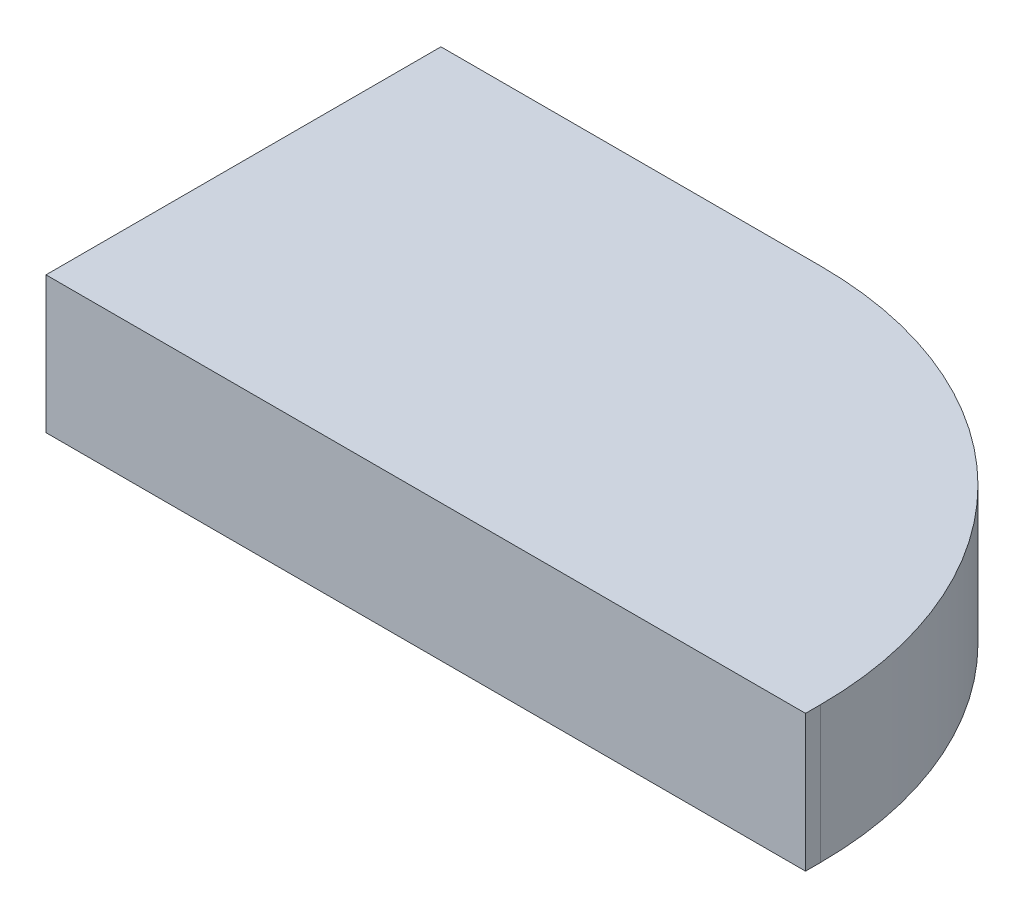
from build123d import *

# Parameters (mm, degrees)
BOSS_EXTRUDE1_DEPTH = 2.25


with BuildPart() as part:
    # Sketch1 → Boss-Extrude1 (new, symmetric)
    with BuildSketch(Plane(origin=(0, 0, 0), x_dir=(1, 0, 0), z_dir=(0, 1, 0))):
        with BuildLine():
            Line((0, 0), (25, 0))
            Line((25, 0), (25, 0.5))
            ThreePointArc((25, 0.5), (21.338834765, 9.338834765), (12.5, 13))
            Line((12.5, 13), (0, 13))
            Line((0, 13), (0, 0))
        make_face()
    extrude(amount=BOSS_EXTRUDE1_DEPTH, both=True)


solid = part.part
